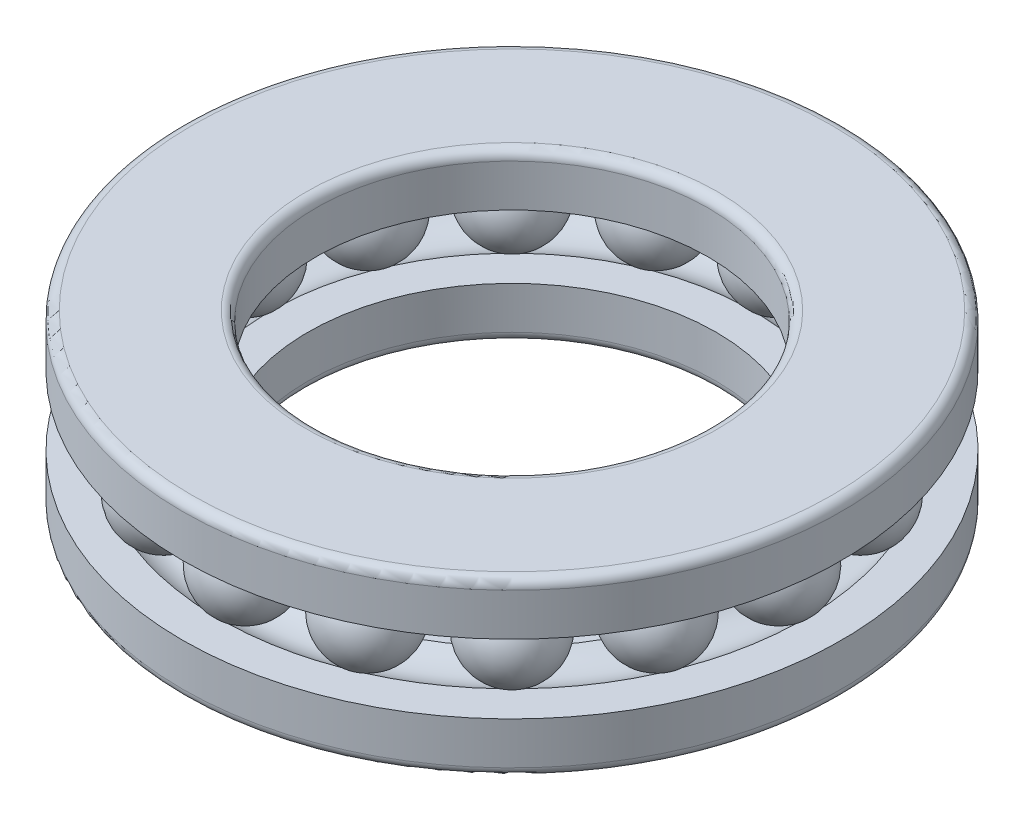
SolidWorks part; units mm, degrees
material "AISI 304"
ref_plane "Plane1" through (0, 0, 0) normal (0, 0, 1) x (1, 0, 0)
ref_plane "Plane2" through (0, 0, 0) normal (0, 1, 0) x (1, 0, 0)
ref_plane "Plane3" through (0, 0, 0) normal (1, 0, 0) x (0, 0, -1)
sketch "Dimension sketch" plane through (0, 0, 0) normal (0, 0, 1) x (1, 0, 0)
  line L0 (0, 0) -> (42, 0)
  point P3 (25, 0)
  point P4 (26, 0)
  point P5 (42, 0)
  point P6 (11, 0)
  point P7 (0.6, 0)
  dimension "DD" = 42
  dimension "d" = 25
  dimension "d1" = 26
  dimension "DD1" = 42
  dimension "T" = 11
  dimension "r" = 0.6
sketch "Sketch1" plane through (0, 0, 0) normal (0, 0, 1) x (1, 0, 0)
  line L0 (21, 0) -> (21, 32.489) construction
  line L1 (0, 0) -> (42, 0)
  line L2 (0, 0) -> (0, 11)
  line L3 (0, 11) -> (42, 11)
  line L4 (42, 0) -> (42, 11)
  line L5 (8.5, 0) -> (8.5, 11)
  line L6 (33.5, 0) -> (33.5, 7.7)
  line L7 (0, 0) -> (0, 11)
  line L8 (42, 0) -> (42, 11)
  line L9 (8, 0) -> (8, 11)
  line L10 (34, 0) -> (34, 11)
  line L11 (0, 5.5) -> (42, 5.5) construction
  line L12 (38, 0) -> (38, 11)
  line L13 (4, 0) -> (4, 11)
  line L14 (0, 3.3) -> (42, 3.3)
  line L15 (0, 7.7) -> (42, 7.7)
  circle A0 centre (4, 5.5) radius 2.75
  dimension "D8" = 5.5
  dimension "D1" = 42
  dimension "D2" = 11
  dimension "D3" = 42
  dimension "D4" = 25
  dimension "D5" = 26
  dimension "D6" = 34
  dimension "D7" = 4.4
sketch "Sketch2" plane through (0, 0, 0) normal (0, 0, 1) x (1, 0, 0)
  line L0 (0, 3.3) -> (42, 3.3) construction
  line L1 (21, 0) -> (21, 32.489) construction
  line L2 (8, 0) -> (8, 11) construction
  line L3 (0, 3.3) -> (2.35, 3.3)
  line L4 (0, 0) -> (42, 0)
  line L5 (42, 0) -> (42, 11)
  line L6 (42, 11) -> (0, 11)
  line L7 (0, 11) -> (0, 0)
  line L8 (0, 0) -> (8, 0)
  line L9 (5.65, 3.3) -> (8, 3.3)
  line L11 (0, 3.3) -> (0, 0)
  line L12 (21, 0) -> (21, 32.489) construction
  line L13 (8, 0) -> (8, 3.3)
  circle A0 centre (4, 5.5) radius 2.75 construction
  arc A1 (2.35, 3.3) -> (5.65, 3.3) centre (4, 5.5) ccw
  dimension "D1" = 0
revolve "Base-Revolve" add sketch "Sketch2" angle 360 about L12
sketch "Sketch3" plane through (0, 0, 0) normal (0, 0, 1) x (1, 0, 0)
  line L2 (4, 0) -> (4, 11) construction
  line L3 (4, 0) -> (4, 11) construction
  line L4 (4, 2.7) -> (4, 8.3)
  circle A0 centre (4, 5.5) radius 2.75 construction
  arc A1 (4, 8.25) -> (4, 2.75) centre (4, 5.5) ccw construction
  arc A2 (4, 8.3) -> (4, 2.7) centre (4, 5.5) ccw
  dimension "D1" = 0.05
revolve "Boss-Revolve2" add sketch "Sketch3" angle 360 about L3
sketch "Sketch4" plane through (0, 0, 0) normal (0, 0, 1) x (1, 0, 0)
  line L0 (21, 0) -> (21, 32.489) construction
  line L1 (0, 7.7) -> (42, 7.7) construction
  line L2 (8.5, 0) -> (8.5, 11) construction
  line L3 (0, 0) -> (0, 11) construction
  line L4 (0, 11) -> (42, 11) construction
  line L5 (21, 0) -> (21, 32.489) construction
  line L6 (0, 7.7) -> (2.35, 7.7)
  line L7 (8.5, 7.7) -> (8.5, 11)
  line L8 (0, 7.7) -> (0, 11)
  line L9 (0, 11) -> (8.5, 11)
  line L12 (5.65, 7.7) -> (8.5, 7.7)
  circle A0 centre (4, 5.5) radius 2.75 construction
  arc A1 (5.65, 7.7) -> (2.35, 7.7) centre (4, 5.5) ccw
revolve "Boss-Revolve3" add sketch "Sketch4" angle 360 about L5
pattern_circular "CirPattern1" count 16 over 360 about axis through (21, 0, 0) along (0, 1, 0) of "Boss-Revolve2"
fillet "Fillet1" radius 0.6 4 edges at (21, 11, -12.5) (21, 11, -21) (21, 0, -13) (21, 0, -21)
